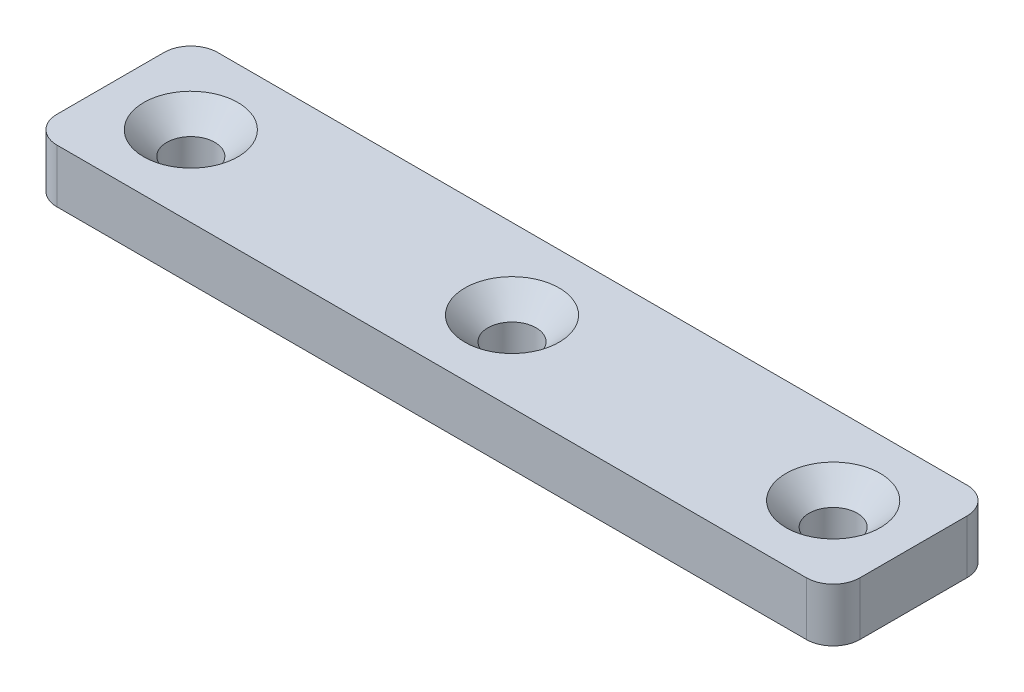
SolidWorks part; units mm, degrees
ref_plane "Front Plane" through (0, 0, 0) normal (0, 0, 1) x (1, 0, 0)
ref_plane "Top Plane" through (0, 0, 0) normal (0, 1, 0) x (1, 0, 0)
ref_plane "Right Plane" through (0, 0, 0) normal (1, 0, 0) x (0, 0, -1)
sketch "Sketch1" plane through (0, 0, 0) normal (0, 1, 0) x (1, 0, 0)
  line L1 (0, 0) -> (150, 0)
  line L2 (0, 0) -> (0, 30)
  line L3 (0, 30) -> (150, 30)
  line L4 (150, 0) -> (150, 30)
  dimension "D1" = 150
  dimension "D2" = 30
extrude "Boss-Extrude1" add sketch "Sketch1" along normal blind 10
fillet "Fillet1" radius 5 4 edges at (0, 5, -30) (150, 5, -30) (150, 5, 0) (0, 5, 0)
sketch "Sketch3" plane through (0, 0, 0) normal (0, -1, 0) x (1, 0, 0)
  line L0 (5, 0) -> (145, 0) construction
  line L1 (0, -25) -> (0, -5) construction
  circle A0 centre (16, -19) radius 11
  circle A1 centre (16, -19) radius 9
  dimension "D1" = 22
  dimension "D2" = 18
  dimension "D3" = 19
  dimension "D4" = 16
extrude "Cut-Extrude2" [suppressed] cut sketch "Sketch3" against normal blind 2
pattern_linear "LPattern1" [suppressed] count 5 spacing 13
pattern_linear "LPattern2" [suppressed] count 7 spacing 28
hole_wizard "Socket Button Head Screw Hole1" positions "Sketch4" profile "Sketch5" countersink size "M8" standard "GB"
sketch "Sketch4" plane through (0, 10, 0) normal (0, 1, 0) x (1, 0, 0)
  line L0 (75, 0) -> (75, 15) construction
  line L1 (5, 0) -> (145, 0) construction
  line L3 (0, 15) -> (15, 15) construction
  line L4 (0, 25) -> (0, 5) construction
  point P0 (75, 15)
  point P2 (15, 15)
  point P4 (135, 15)
  dimension "D1" = 120
sketch "Sketch5" plane through (75, 10, -15) normal (1, 0, 0) x (0, 0, 1)
  line L0 (0, 0) -> (0, 22.4539)
  line L1 (0, 22.4539) -> (4.5, 19.75)
  line L2 (4.5, 19.75) -> (4.5, 4.3)
  line L3 (4.5, 4.3) -> (8.8, 0)
  line L5 (8.8, 0) -> (0, 0)
  line L6 (-4.5, 4.3) -> (-8.8, 0) construction
  line L10 (0, 22.4539) -> (-4.5, 19.75) construction
  line L11 (0, -6.35) -> (0, 107.95) construction
  dimension "孔直径" = 9
  dimension "孔深度" = 19.75
  dimension "近端锥形沉头孔直径" = 17.6
  dimension "近端锥形沉头孔角度" = 90
  dimension "导头角度" = 118
